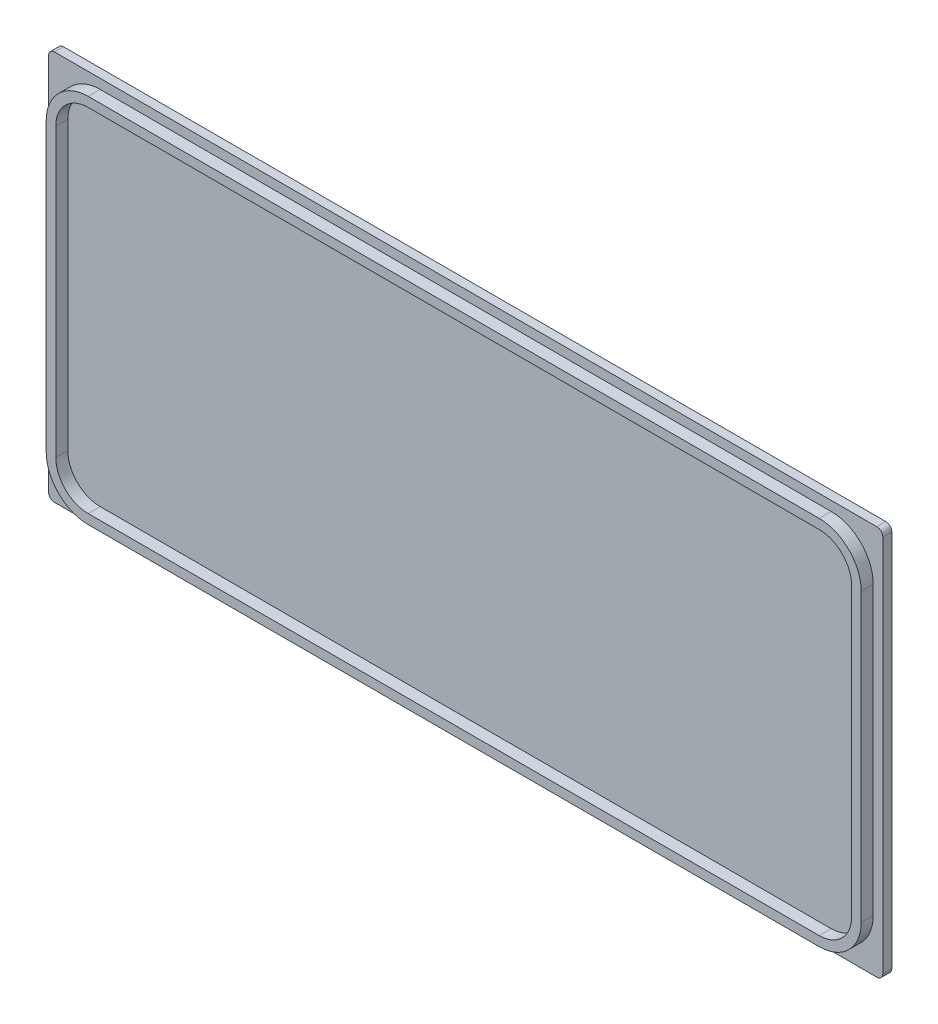
from build123d import *

# Parameters (mm, degrees)
BOSS_EXTRUDE1_DEPTH = 1.5
BOSS_EXTRUDE2_START = -1.5
SKETCH2_R           = 6
SKETCH2_R_2         = 5.1
BOSS_EXTRUDE2_DEPTH = 1
BOSS_EXTRUDE3_DEPTH = 2
SKETCH7_W           = 2
SKETCH7_H           = 19.411603012
CUT_EXTRUDE3_DEPTH  = 0.8
CUT_EXTRUDE4_START  = -1
SKETCH8_R           = 5.1
CUT_EXTRUDE4_DEPTH  = 1


with BuildPart() as part:
    # Sketch1 → Boss-Extrude1 (new body)
    with BuildSketch(Plane.XY):
        with BuildLine():
            Line((-68.5, 32.5), (68.5, 32.5))
            ThreePointArc((68.5, 32.5), (69.207106781, 32.207106781), (69.5, 31.5))
            Line((69.5, 31.5), (69.5, -31.5))
            ThreePointArc((69.5, -31.5), (69.207106781, -32.207106781), (68.5, -32.5))
            Line((68.5, -32.5), (-68.5, -32.5))
            ThreePointArc((-68.5, -32.5), (-69.207106781, -32.207106781), (-69.5, -31.5))
            Line((-69.5, -31.5), (-69.5, 31.5))
            ThreePointArc((-69.5, 31.5), (-69.207106781, 32.207106781), (-68.5, 32.5))
        make_face()
    extrude(amount=BOSS_EXTRUDE1_DEPTH)

    # Sketch2 → Boss-Extrude2 (add)
    # profile 1 of 4: a face of its own
    with BuildSketch(Plane.XY.offset(1.5).offset(BOSS_EXTRUDE2_START)):
        with Locations((-58, 18)):
            Circle(SKETCH2_R)
        with Locations((-58, 18)):
            Circle(SKETCH2_R_2, mode=Mode.SUBTRACT)
    # profile 2 of 4: a face of its own
    with BuildSketch(Plane.XY.offset(1.5).offset(BOSS_EXTRUDE2_START)):
        with Locations((58, 18)):
            Circle(SKETCH2_R)
        with Locations((58, 18)):
            Circle(SKETCH2_R_2, mode=Mode.SUBTRACT)
    # profile 3 of 4: a face of its own
    with BuildSketch(Plane.XY.offset(1.5).offset(BOSS_EXTRUDE2_START)):
        with Locations((-58, -18)):
            Circle(SKETCH2_R)
        with Locations((-58, -18)):
            Circle(SKETCH2_R_2, mode=Mode.SUBTRACT)
    # profile 4 of 4: a face of its own
    with BuildSketch(Plane.XY.offset(1.5).offset(BOSS_EXTRUDE2_START)):
        with Locations((58, -18)):
            Circle(SKETCH2_R)
        with Locations((58, -18)):
            Circle(SKETCH2_R_2, mode=Mode.SUBTRACT)
    extrude(amount=-BOSS_EXTRUDE2_DEPTH)

    # Sketch3 → Boss-Extrude3 (add)
    with BuildSketch(Plane.XY.offset(1.5)):
        with BuildLine():
            Line((60.9, 30.9), (-60.9, 30.9))
            ThreePointArc((-60.9, 30.9), (-65.849747468, 28.849747468), (-67.9, 23.9))
            Line((-67.9, 23.9), (-67.9, -23.9))
            ThreePointArc((-67.9, -23.9), (-65.849747468, -28.849747468), (-60.9, -30.9))
            Line((-60.9, -30.9), (60.9, -30.9))
            ThreePointArc((60.9, -30.9), (65.849747468, -28.849747468), (67.9, -23.9))
            Line((67.9, -23.9), (67.9, 23.9))
            ThreePointArc((67.9, 23.9), (65.849747468, 28.849747468), (60.9, 30.9))
        make_face()
        with BuildLine():
            Line((60.9, 29.3), (-60.9, 29.3))
            ThreePointArc((-60.9, 29.3), (-64.718376618, 27.718376618), (-66.3, 23.9))
            Line((-66.3, 23.9), (-66.3, -23.9))
            ThreePointArc((-66.3, -23.9), (-64.718376618, -27.718376618), (-60.9, -29.3))
            Line((-60.9, -29.3), (60.9, -29.3))
            ThreePointArc((60.9, -29.3), (64.718376618, -27.718376618), (66.3, -23.9))
            Line((66.3, -23.9), (66.3, 23.9))
            ThreePointArc((66.3, 23.9), (64.718376618, 27.718376618), (60.9, 29.3))
        make_face(mode=Mode.SUBTRACT)
    extrude(amount=BOSS_EXTRUDE3_DEPTH)

    # Sketch7 → Cut-Extrude3 (cut)
    with BuildSketch(Plane(origin=(0, -32.5, 0), x_dir=(-1, 0, 0), z_dir=(0, -1, 0))):
        Rectangle(SKETCH7_W, SKETCH7_H)
    extrude(amount=-CUT_EXTRUDE3_DEPTH, mode=Mode.SUBTRACT)

    # Sketch8 → Cut-Extrude4 (cut)
    with BuildSketch(Plane(origin=(0, 0, 0), x_dir=(-1, 0, 0), z_dir=(0, 0, -1)).offset(CUT_EXTRUDE4_START)):
        with Locations(Location((-58, 18, 0), (0, 0, 180))):
            Circle(SKETCH8_R)
        with Locations(Location((58, 18, 0), (0, 0, 180))):
            Circle(SKETCH8_R)
        with Locations(Location((58, -18, 0), (0, 0, 180))):
            Circle(SKETCH8_R)
        with Locations(Location((-58, -18, 0), (0, 0, 180))):
            Circle(SKETCH8_R)
    extrude(amount=CUT_EXTRUDE4_DEPTH, mode=Mode.SUBTRACT)


solid = part.part
